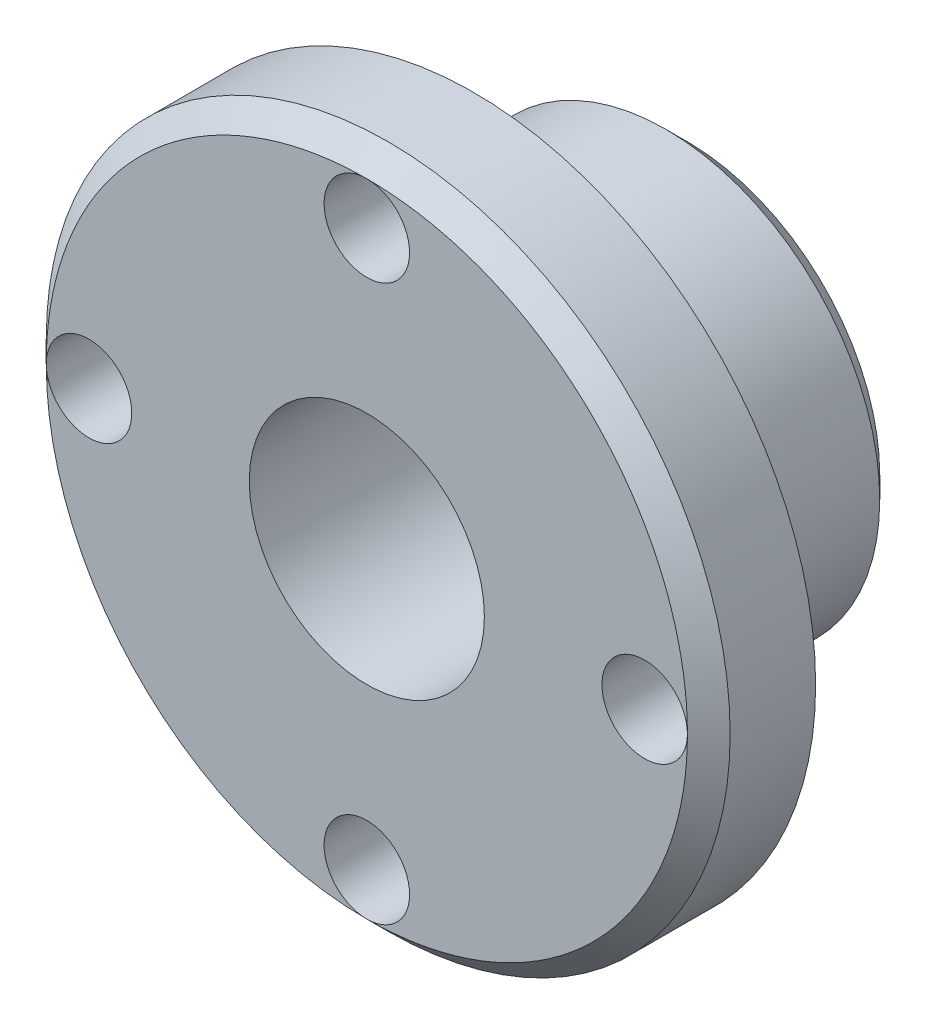
from build123d import *

# Parameters (mm, degrees)
SKETCH1_R           = 10
BOSS_EXTRUDE1_DEPTH = 10
SKETCH2_R           = 16
BOSS_EXTRUDE2_DEPTH = 5
CHAMFER1_SIZE       = 1
SKETCH3_R           = 2
CUT_EXTRUDE1_DEPTH  = 10
CIRPATTERN1_COUNT   = 4
SKETCH4_R           = 5.5
CUT_EXTRUDE2_DEPTH  = 29


with BuildPart() as part:
    # Sketch1 → Boss-Extrude1 (new body)
    with BuildSketch(Plane.XY):
        Circle(SKETCH1_R)
    extrude(amount=BOSS_EXTRUDE1_DEPTH)

    # Sketch2 → Boss-Extrude2 (add)
    with BuildSketch(Plane.XY.offset(10)):
        Circle(SKETCH2_R)
    extrude(amount=BOSS_EXTRUDE2_DEPTH)

    # Chamfer1
    chamfer1_edges = [part.edges().sort_by_distance(p)[0] for p in [
        (-10, 0, 0),
        (-16, 0, 15),
    ]]
    chamfer(chamfer1_edges, length=CHAMFER1_SIZE)

    # Sketch3 → Cut-Extrude1 (cut)
    with BuildSketch(Plane(origin=(0, 0, 10), x_dir=(-1, 0, 0), z_dir=(0, 0, -1))):
        with Locations((0, 13)):
            Circle(SKETCH3_R)
    cut_extrude1 = extrude(amount=-CUT_EXTRUDE1_DEPTH, mode=Mode.SUBTRACT)

    # CirPattern1: Cut-Extrude1 ×4 about axis
    cirpattern1_axis = Axis((0, 0, 0), (0, 0, 1))
    for i in range(1, CIRPATTERN1_COUNT):
        add(cut_extrude1.rotate(cirpattern1_axis, i * 360 / CIRPATTERN1_COUNT), mode=Mode.SUBTRACT)

    # Sketch4 → Cut-Extrude2 (cut)
    with BuildSketch(Plane(origin=(0, 0, 0), x_dir=(-1, 0, 0), z_dir=(0, 0, -1))):
        Circle(SKETCH4_R)
    extrude(amount=-CUT_EXTRUDE2_DEPTH, mode=Mode.SUBTRACT)


solid = part.part
